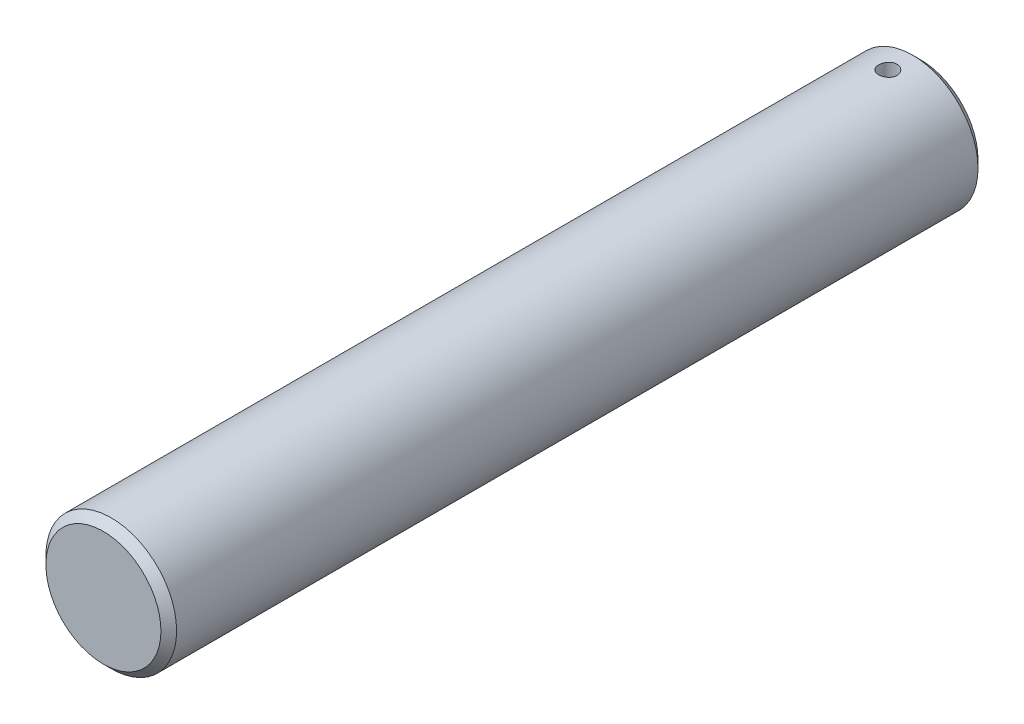
from build123d import *

# Parameters (mm, degrees)
SKETCH1_R               = 12.7
BOSS_EXTRUDE1_DEPTH     = 158.75
CHAMFER1_SIZE           = 1.524
CUT_EXTRUDE1_DEPTH      = 160.762769443
CUT_EXTRUDE1_DEPTH_BACK = 160.762769443
SKETCH2_R               = 1.785


with BuildPart() as part:
    # Sketch1 → Boss-Extrude1 (new body)
    with BuildSketch(Plane.XY):
        with Locations(Location((0, 0, 0), (0, 0, 180))):
            Circle(SKETCH1_R)
    extrude(amount=BOSS_EXTRUDE1_DEPTH)

    # Chamfer1
    chamfer1_edges = [part.edges().sort_by_distance(p)[0] for p in [
        (12.7, 0, 0),
        (12.7, 0, 158.75),
    ]]
    chamfer(chamfer1_edges, length=CHAMFER1_SIZE)

    # Sketch2 → Cut-Extrude1 (cut, two sides: drawn at the far end of the back side and taken through both)
    with BuildSketch(Plane(origin=(0, 0, 0), x_dir=(1, 0, 0), z_dir=(0, 1, 0)).offset(-CUT_EXTRUDE1_DEPTH_BACK)):
        with Locations(Location((0, -6.35, 0), (0, 0, 270))):
            Circle(SKETCH2_R)
    extrude(amount=CUT_EXTRUDE1_DEPTH + CUT_EXTRUDE1_DEPTH_BACK, mode=Mode.SUBTRACT)


solid = part.part
